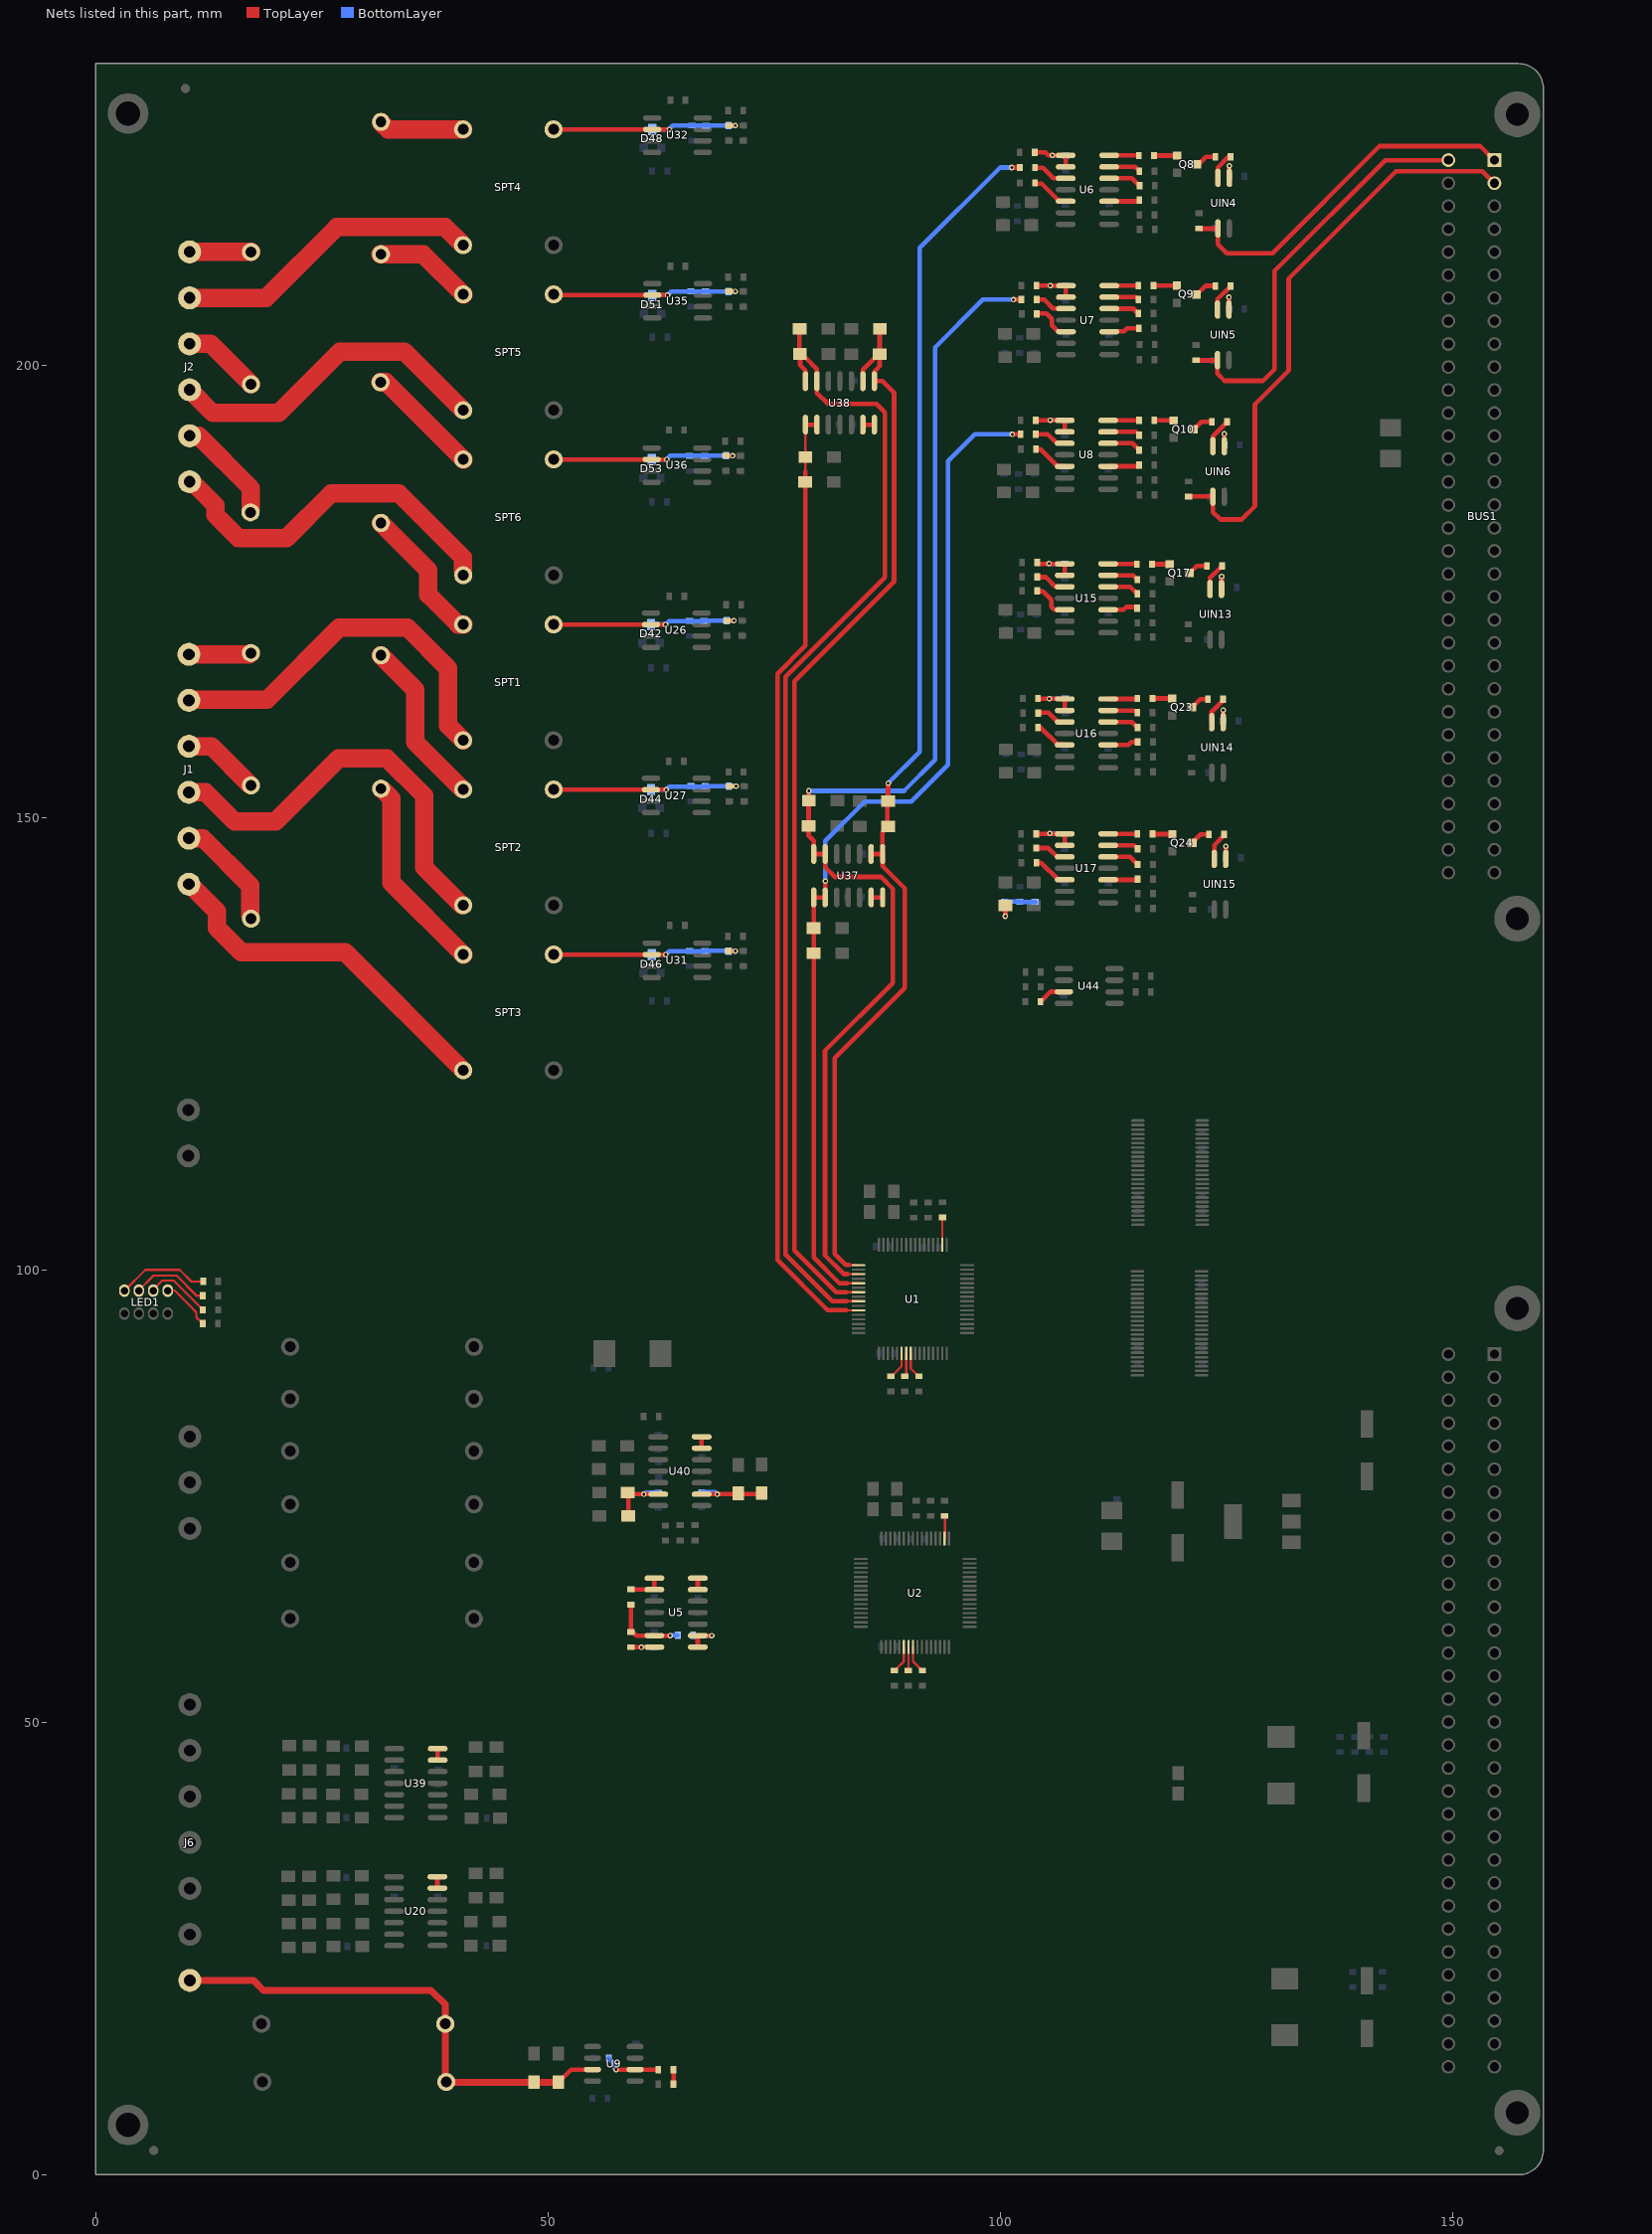
[diagram p0: the nets of this part, all layers, seen from the top]
# Altium PCB MISC80584.PCBDoc (part 6 of 7)
Units mm, origin at the board's own origin, x right, y up, seen from the top; angles counter-clockwise.
Board outline 160.02 x 233.3 mm, 4 copper layers (TopLayer, GND, POWER, BottomLayer); 386 components, 266 nets, 1374 pads, 640 vias.

## Via types
v1: diameter 0.61, hole 0.305, TopLayer to BottomLayer, 342 vias
v2: diameter 0.762, hole 0.381, TopLayer to BottomLayer, 197 vias
v3: diameter 0.508, hole 0.254, TopLayer to BottomLayer, 101 vias

## Nets (pads, with @x,y where several pads share a name; then routed paths per layer and width w, separated by ;. In a path a pad name is that pad's centre, name@x,y a point inside that pad or via, vN(x,y) a via of type N, cw(c..) or ccw(c..) an arc to the next point about the centre after c; other vN are vias at no path point) (continued)
NetD91_A: D91.A R359.1 R366.2 R374.2 | length 6.2
  TopLayer w0.508: v1(100.559,139.116) D91.A@100.559,140.284
  BottomLayer w0.508: v1@100.559,139.167 100.559,140.64 R359.1@100.482,140.716 R374.2@102.159,140.716 102.184,140.716 102.235,140.665 R366.2@103.886,140.665
NetD94_A: D94.A D96.K R93.2 U40.6 | length 7.1
  TopLayer w0.508: D94.A@58.903,73.05 58.903,75.159 59.004,75.26 59.03,75.235 60.528,75.235 v1(60.604,75.235) U40.6@62.192,75.235
  BottomLayer w0.508: v1@60.63,75.235 60.808,75.413 R93.2@62.179,75.413
NetD95_A: D95.A D97.K R85.2 U40.9 | length 8.4
  TopLayer w0.508: U40.9@66.992,75.235 v1(68.707,75.235) ; v1@68.758,75.235 D97.K@73.635,75.235
  BottomLayer w0.508: R85.2@67.005,75.463 68.453,75.463 v1@68.707,75.209
NetLED1_1: LED1.1 R339.1 | length 10.1
  TopLayer w0.254: LED1.1@3.175,97.739 3.226,97.739 5.512,100.025 9.296,100.025 10.592,98.73 R339.1@11.836,98.73
NetLED1_3: LED1.3 R342.1 | length 8.8
  TopLayer w0.254: LED1.3@4.674,97.663 6.401,99.39 8.966,99.39 11.201,97.155 R342.1@11.811,97.155
NetLED1_5: LED1.5 R340.1 | length 6.9
  TopLayer w0.254: LED1.5@6.477,97.942 7.379,98.844 8.623,98.844 R340.1@11.735,95.733
NetLED1_7: LED1.7 R341.1 | length 5.7
  TopLayer w0.254: LED1.7@7.975,97.739 8.738,97.739 10.389,96.088 11.138,95.339 11.138,94.78 11.76,94.158 R341.1@11.76,94.056
NetQ8_B: Q8.B R162.1 | length 2.4
  TopLayer w0.508: R162.1@117.145,223.164 Q8.B@119.558,223.164
NetQ8_C: Q8.C R491.2 | length 2.1
  TopLayer w0.508: Q8.C@121.996,222.301 122.733,223.037 R491.2@123.774,223.037
NetQ9_B: Q9.B R211.1 | length 2.5
  TopLayer w0.508: R211.1@116.992,208.788 Q9.B@119.507,208.788
NetQ9_C: Q9.C R492.2 | length 2.2
  TopLayer w0.508: Q9.C@121.92,208.001 122.682,208.763 R492.2@123.774,208.763
NetQ10_B: Q10.B R225.1 | length 1.9
  TopLayer w0.508: R225.1@117.018,193.904 Q10.B@118.923,193.904
NetQ10_C: Q10.C R493.2 | length 2.3
  TopLayer w0.508: Q10.C@121.437,192.938 122.225,193.726 R493.2@123.393,193.726
NetQ17_B: Q17.B R382.1 | length 1.8
  TopLayer w0.508: R382.1@116.764,178.003 Q17.B@118.542,178.003
NetQ17_C: Q17.C R510.2 | length 1.9
  TopLayer w0.508: Q17.C@121.133,177.241 121.717,177.825 R510.2@122.834,177.825
NetQ23_B: Q23.B R383.1 | length 2.1
  TopLayer w0.508: R383.1@116.865,163.144 116.891,163.17 Q23.B@118.999,163.17
NetQ23_C: Q23.C R511.2 | length 1.9
  TopLayer w0.508: Q23.C@121.387,162.382 122.098,163.093 R511.2@122.961,163.093
NetQ24_B: Q24.B R384.1 | length 2.1
  TopLayer w0.508: R384.1@116.967,148.184 Q24.B@119.024,148.184
NetQ24_C: Q24.C R512.2 | length 2.3
  TopLayer w0.508: Q24.C@121.183,147.218 122.123,148.158 123.012,148.158 R512.2@123.063,148.107
NetR10_1: R10.1 R12.1 R13.2 U5.6 | length 8
  TopLayer w0.508: R13.2@59.182,60.02 R10.1@59.182,62.916 ; R13.2@59.36,60.02 59.766,59.614 U5.6@61.76,59.614 v1(63.5,59.614)
  BottomLayer w0.508: v1(63.5,59.614) 63.525,59.639 R12.1@64.313,59.639
NetR10_2: R10.2 U5.1 U5.2 | length 3.7
  TopLayer w0.508: R10.2@59.233,64.694 U5.2@61.76,64.694 U5.1@61.76,65.824
NetR11_1: R11.1 R14.2 U9.6 | length 6.2
  TopLayer w0.508: v1(57.531,11.659) U9.6@59.627,11.659 R14.2@62.103,11.659
  BottomLayer w0.508: R11.1@56.693,12.929 57.379,12.243 57.379,11.811 v1(57.531,11.659)
NetR12_2: R12.2 U5.8 U5.9 | length 4.6
  TopLayer w0.508: U5.8@66.56,58.344 U5.9@66.56,59.448 ; U5.9@66.56,59.614 v1(68.097,59.614)
  BottomLayer w0.508: R12.2@66.167,59.614 66.192,59.588 68.123,59.588 v1(68.097,59.614)
NetR13_1: R13.1 R28.2 U5.7 | length 3.3
  TopLayer w0.508: R13.1@59.182,58.344 U5.7@61.036,58.344
  BottomLayer w0.508: v1(60.325,58.318) 60.35,58.344 R28.2@61.747,58.344
NetR33_1: R33.1 U1.34 | length 2.8
  TopLayer w0.254: U1.34@93.589,102.805 R33.1@93.589,105.603
NetR34_1: R34.1 U2.34 | length 2.5
  TopLayer w0.254: U2.34@93.843,70.344 93.891,70.392 93.891,72.763 R34.1@93.843,72.811
NetR37_1: R37.1 U6.3 | length 3.7
  TopLayer w0.508: R37.1@103.962,221.818 104.699,221.818 105.867,220.65 U6.3@107.226,220.65
NetR40_1: R40.1 U7.3 | length 3
  TopLayer w0.508: R40.1@104.013,207.239 104.851,207.239 105.816,206.273 U7.3@106.578,206.273
NetR48_1: R48.1 U8.3 | length 3.5
  TopLayer w0.508: R48.1@104.013,192.38 105.232,192.38 106.248,191.364 U8.3@107.125,191.364
NetR57_2: R57.2 R76.2 U6.1 U6.2 | length 6.1
  TopLayer w0.508: R57.2@103.861,223.52 104.978,223.52 105.308,223.19 v1(105.766,223.19) 105.791,223.19 107.087,223.19 107.226,223.05 U6.2@107.226,221.92
  BottomLayer w0.508: v1(105.766,223.19) R76.2@107.188,223.19
NetR58_2: R58.2 R86.2 U7.1 U7.2 | length 6.1
  TopLayer w0.508: R58.2@103.988,208.839 104.038,208.788 v1(105.512,208.788) U7.1@107.252,208.788 ; U7.1@107.239,208.737 107.252,208.725 U7.2@107.252,207.518
  BottomLayer w0.508: v1@105.613,208.788 R86.2@107.213,208.788
NetR59_2: R59.2 R87.2 U8.1 U8.2 | length 5.9
  TopLayer w0.508: R59.2@104.115,193.904 v1@105.512,193.904 ; v1(105.512,193.929) v1@105.512,193.904 ; U8.2@107.125,192.634 U8.1@107.125,193.814 ; U8.1@107.125,193.904 v1@105.512,193.904
  BottomLayer w0.508: v1@105.588,193.904 R87.2@107.112,193.904 R87.2@107.239,193.904
NetR145_1: R145.1 SPT1.0 | length 15.3
  TopLayer w2.032: R145.1@31.545,182.565 36.779,177.33 36.779,174.65 40.081,171.348 SPT1.0@40.665,171.348
NetR150_1: R150.1 U6.13 | length 3.5
  TopLayer w0.508: U6.13@112.026,221.92 114.884,221.92 R150.1@115.341,221.463
NetR151_1: R151.1 U7.13 | length 3.3
  TopLayer w0.508: U7.13@112.052,207.518 114.986,207.518 R151.1@115.214,207.289
NetR152_1: R152.1 U8.13 | length 3.6
  TopLayer w0.508: U8.13@111.925,192.634 115.011,192.634 R152.1@115.367,192.278
NetR155_1: R155.1 U6.12 | length 3.6
  TopLayer w0.508: U6.12@112.026,220.65 114.554,220.65 R155.1@115.316,219.888
NetR156_1: R156.1 U7.12 | length 3.3
  TopLayer w0.508: U7.12@112.052,206.248 114.706,206.248 R156.1@115.164,205.791
NetR157_1: R157.1 U8.12 | length 3.6
  TopLayer w0.508: U8.12@111.925,191.364 114.605,191.364 R157.1@115.24,190.729
NetR161_1: R161.1 SPT2.0 | length 18.2
  TopLayer w2.032: R161.1@31.545,167.934 35.331,164.147 35.331,158.344 SPT2.0@40.335,153.34
NetR162_2: R162.2 U6.14 | length 3.2
  TopLayer w0.508: U6.14@112.026,223.19 R162.2@115.24,223.19
NetR165_1: R165.1 SPT3.0 | length 21.8
  TopLayer w2.032: R165.1@31.775,153.035 32.69,152.121 32.69,142.823 SPT3.0@40.64,134.872
NetR168_1: R168.1 SPT4.0 | length 9.3
  TopLayer w2.032: R168.1@31.598,226.771 32.31,226.058 SPT4.0@40.615,226.058
NetR171_1: R171.1 SPT5.0 | length 11
  TopLayer w2.032: R171.1@31.496,212.268 36.193,212.268 SPT5.0@40.64,207.821
NetR174_1: R174.1 SPT6.0 | length 12.7
  TopLayer w2.032: R174.1@31.471,198.12 32.104,198.12 SPT6.0@40.64,189.584
NetR211_2: R211.2 U7.14 | length 3.1
  TopLayer w0.508: U7.14@112.052,208.788 R211.2@115.164,208.788
NetR224_1: R224.1 U44.3 | length 2.8
  TopLayer w0.508: R224.1@104.597,129.819 105.537,130.759 U44.3@107.036,130.759
NetR225_2: R225.2 U8.14 | length 3.3
  TopLayer w0.508: U8.14@111.925,193.904 R225.2@115.265,193.904
NetR349_1: R349.1 U15.3 | length 3.5
  TopLayer w0.508: R349.1@104.089,176.581 105.029,176.581 106.096,175.514 U15.3@107.125,175.514
NetR350_1: R350.1 U16.3 | length 3.1
  TopLayer w0.508: R350.1@104.496,161.595 105.334,161.595 106.35,160.579 U16.3@107.125,160.579
NetR351_1: R351.1 U17.3 | length 3.4
  TopLayer w0.508: R351.1@104.14,146.634 105.308,146.634 106.274,145.669 U17.3@107.125,145.669
NetR353_2: R353.2 R360.2 U15.1 U15.2 | length 5.9
  TopLayer w0.508: R353.2@104.038,178.054 v1@105.385,178.054 ; v1(105.385,178.079) v1@105.385,178.054 ; U15.2@107.125,176.784 U15.1@107.125,177.965 ; U15.1@107.125,178.054 v1@105.385,178.054
  BottomLayer w0.508: v1@105.512,178.054 R360.2@107.112,178.054
NetR354_2: R354.2 R361.2 U16.1 U16.2 | length 5.5
  TopLayer w0.508: R354.2@104.369,163.144 v1(105.41,163.144) 105.537,163.144 U16.1@106.731,163.144 ; U16.1@106.731,163.119 U16.1@107.125,163.119 U16.2@107.125,161.912
  BottomLayer w0.508: v1(105.41,163.144) R361.2@106.985,163.144
NetR355_2: R355.2 R362.2 U17.1 U17.2 | length 5.8
  TopLayer w0.508: R355.2@104.178,148.221 v1@105.486,148.221 ; v1(105.486,148.26) v1@105.486,148.221 ; U17.2@107.125,146.939 U17.1@107.125,148.209 107.125,148.221 v1@105.486,148.221
  BottomLayer w0.508: v1(105.486,148.26) R362.2@107.01,148.26
NetR375_1: R375.1 U15.13 | length 3.4
  TopLayer w0.508: U15.13@111.925,176.784 114.681,176.784 R375.1@115.113,176.352
NetR376_1: R376.1 U16.13 | length 3.2
  TopLayer w0.508: U16.13@111.925,161.849 114.757,161.849 R376.1@115.011,161.595
NetR377_1: R377.1 U17.13 | length 3.4
  TopLayer w0.508: U17.13@111.925,146.939 114.757,146.939 R377.1@115.138,146.558
NetR379_1: R379.1 U15.12 | length 3.5
  TopLayer w0.508: U15.12@111.925,175.514 114.351,175.514 R379.1@115.087,174.777
NetR380_1: R380.1 U16.12 | length 3.3
  TopLayer w0.508: U16.12@111.925,160.579 114.554,160.579 R380.1@115.062,160.071
NetR381_1: R381.1 U17.12 | length 3.6
  TopLayer w0.508: U17.12@111.925,145.669 114.325,145.669 R381.1@115.138,144.856
NetR382_2: R382.2 U15.14 | length 3
  TopLayer w0.508: U15.14@111.925,178.054 R382.2@114.91,178.054
NetR383_2: R383.2 U16.14 | length 3.2
  TopLayer w0.508: U16.14@111.925,163.119 115.087,163.119 R383.2@115.113,163.144
NetR384_2: R384.2 U17.14 | length 3.1
  TopLayer w0.508: U17.14@111.925,148.209 R384.2@115.037,148.209
NetR399_1: R399.1 U6.5 | length 4.1
  TopLayer w0.508: R399.1@103.911,220.04 104.572,220.04 106.502,218.11 U6.5@107.226,218.11
NetR400_1: R400.1 U7.5 | length 4.5
  TopLayer w0.508: R400.1@103.988,205.74 104.013,205.715 105.105,205.715 105.689,205.13 105.689,204.419 106.401,203.708 U7.5@107.252,203.708
NetR401_1: R401.1 U8.5 | length 3.8
  TopLayer w0.508: R401.1@104.089,190.729 104.445,190.729 106.324,188.849 U8.5@107.086,188.849 ; U8.5@107.086,188.824 U8.5@107.125,188.824
NetR423_1: R423.1 U15.5 | length 4.3
  TopLayer w0.508: R423.1@104.064,175.031 R423.1@104.191,175.031 ; R423.1@104.191,174.955 R423.1@104.216,174.955 ; R423.1@104.216,175.006 104.724,175.006 105.644,174.086 105.644,173.324 105.994,172.974 U15.5@107.125,172.974
NetR430_1: R430.1 U16.5 | length 3.7
  TopLayer w0.508: R430.1@104.292,159.995 104.394,159.995 105.435,158.953 105.461,158.953 106.35,158.064 U16.5@107.188,158.064
NetR431_1: R431.1 U17.5 | length 3.9
  TopLayer w0.508: R431.1@104.064,145.009 R431.1@104.089,145.009 ; R431.1@104.089,145.034 104.496,145.034 106.401,143.129 U17.5@107.125,143.129
NetR435_1: R435.1 U8.10 | length 3.3
  TopLayer w0.508: U8.10@111.925,188.824 R435.1@115.24,188.824
NetR437_1: R437.1 U6.10 | length 3.3
  TopLayer w0.508: U6.10@112.026,218.11 R437.1@115.316,218.11
NetR438_1: R438.1 U7.10 | length 3.4
  TopLayer w0.508: U7.10@112.052,203.708 112.077,203.733 113.665,203.733 113.995,204.064 R438.1@115.291,204.064
NetR444_1: R444.1 U15.10 | length 3.3
  TopLayer w0.508: U15.10@111.925,172.974 113.64,172.974 113.944,173.279 R444.1@115.113,173.279
NetR445_1: R445.1 U16.10 | length 3.4
  TopLayer w0.508: U16.10@111.925,158.039 114.148,158.039 114.478,158.369 R445.1@115.189,158.369
NetR446_1: R446.1 U17.10 | length 3.2
  TopLayer w0.508: U17.10@111.925,143.129 R446.1@115.087,143.129
NetR486_2: R486.2 UIN4.1 | length 2.5
  TopLayer w0.508: UIN4.1@125.324,220.701 v1(125.324,222.047)
  BottomLayer w0.508: R486.2@125.324,220.929 v1(125.324,222.047)
NetR487_2: R487.2 UIN5.1 | length 2.6
  TopLayer w0.508: UIN5.1@125.273,206.146 v1(125.273,207.518)
  BottomLayer w0.508: v1@125.273,207.467 125.273,206.248 R487.2@125.298,206.223
NetR488_2: R488.2 UIN6.1 | length 2.6
  TopLayer w0.508: UIN6.1@124.765,191.059 124.765,192.43 v1(124.765,192.405)
  BottomLayer w0.508: R488.2@124.739,191.313 124.765,191.338 124.765,192.43 v1(124.765,192.405)
NetR491_1: R491.1 UIN4.2 | length 3.1
  TopLayer w0.508: UIN4.2@124.054,220.701 124.054,221.844 125.273,223.063 R491.1@125.527,223.063
NetR492_1: R492.1 UIN5.2 | length 3
  TopLayer w0.508: UIN5.2@124.003,206.146 124.003,207.289 R492.1@125.349,208.636
NetR493_1: R493.1 UIN6.2 | length 3.4
  TopLayer w0.508: UIN6.2@123.495,191.059 123.495,192.13 125.09,193.726 R493.1@125.12,193.726
NetR503_2: R503.2 UIN13.1 | length 2.6
  TopLayer w0.508: UIN13.1@124.46,175.26 v1(124.46,176.657)
  BottomLayer w0.508: R503.2@124.46,175.463 v1(124.46,176.657)
NetR506_2: R506.2 UIN14.1 | length 2.6
  TopLayer w0.508: UIN14.1@124.638,160.553 v1(124.638,161.874)
  BottomLayer w0.508: v1(124.638,161.874) 124.638,160.68 R506.2@124.689,160.63
NetR507_2: R507.2 UIN15.1 | length 2.6
  TopLayer w0.508: UIN15.1@124.917,145.44 v1(124.917,146.837)
  BottomLayer w0.508: R507.2@124.917,145.618 v1(124.917,146.837)
NetR510_1: R510.1 UIN13.2 | length 2.8
  TopLayer w0.508: UIN13.2@123.19,175.26 123.19,176.505 R510.1@124.308,177.622
NetR511_1: R511.1 UIN14.2 | length 2.9
  TopLayer w0.508: UIN14.2@123.368,160.553 123.368,161.696 R511.1@124.638,162.966
NetR512_1: R512.1 UIN15.2 | length 2.9
  TopLayer w0.508: UIN15.2@123.647,145.44 123.647,146.964 R512.1@124.612,147.93
NetR605_1: R605.1 U1.8 | length 2.7
  TopLayer w0.254: U1.8@90.089,90.805 90.089,89.134 R605.1@90.805,88.417 ; R605.1@90.983,88.367 R605.1@90.983,88.417
NetR607_1: R607.1 U1.7 | length 2.5
  TopLayer w0.254: R607.1@89.56,88.341 89.589,88.369 U1.7@89.589,90.805
NetR608_1: R608.1 U1.6 | length 2.7
  TopLayer w0.254: R608.1@88.163,88.443 89.089,89.368 U1.6@89.089,90.805
NetR609_1: R609.1 U2.8 | length 2.9
  TopLayer w0.254: U2.8@90.343,58.344 90.343,56.774 R609.1@91.288,55.829
NetR611_1: R611.1 U2.7 | length 2.4
  TopLayer w0.254: R611.1@89.843,55.979 U2.7@89.843,58.344
NetR612_1: R612.1 U2.6 | length 2.8
  TopLayer w0.254: R612.1@88.443,55.88 89.343,56.78 U2.6@89.343,58.344
NetU5_13: U5.13 U5.14 | length 1.3
  TopLayer w0.508: U5.14@66.599,65.888 66.56,65.849 U5.13@66.56,64.694 U5.13@66.65,64.783
NetU20_13: U20.13 U20.14 | length 1.3
  TopLayer w0.508: U20.14@37.744,32.969 37.782,32.931 U20.13@37.782,31.699
NetU37_13: U37.13 U37.14 | length 1.3
  TopLayer w0.508: U37.13@85.725,141.186 86.931,141.186 U37.14@86.995,141.122
NetU38_13: U38.13 U38.14 | length 1.1
  TopLayer w0.508: U38.13@85.027,193.434 U38.14@86.081,193.434
NetU39_13: U39.13 U39.14 | length 1.2
  TopLayer w0.508: U39.14@37.77,47.041 37.808,47.003 U39.13@37.808,45.847
NetU40_13: U40.13 U40.14 | length 1
  TopLayer w0.508: U40.13@66.992,80.556 U40.14@66.992,81.585
U1+: J2.1 R168.2 | length 6.8
  TopLayer w2.032: J2.1@10.389,212.522 R168.2@17.196,212.522
U1-: J2.2 SPT4.1 | length 34
  TopLayer w2.032: J2.2@10.389,207.442 18.847,207.442 26.67,215.265 38.633,215.265 SPT4.1@40.437,213.462
U1I: D10.A D14.K U1.55 U38.1 U38.2 | length 120.1
  TopLayer w0.254: 82.956,97.555 U1.55@84.339,97.555
  TopLayer w0.508: 82.956,97.561 81.864,97.561 77.241,102.184 77.241,165.075 88.265,176.098 88.265,196.926 86.957,198.234 U38.1@86.081,198.234 86.081,199.314 86.665,199.898 D10.A@86.665,201.219 86.665,203.784 D14.K@86.792,203.911 ; U38.2@84.811,198.234 84.811,199.517 D10.A@86.081,200.787
U1IN: C104.2 D48.3 R118.2 R119.2 R120.2 SPT4.3 U32.2 | length 22.7
  TopLayer w0.508: SPT4.3@50.597,226.06 U32.2@61.519,226.06 v1(63.424,226.06) ; C104.2@69.977,226.492 v1(70.714,226.492)
  BottomLayer w0.508: D48.3@61.544,226.06 63.373,226.06 63.779,226.466 R119.2@67.488,226.466 69.825,226.466 R118.2@69.85,226.492 ; R118.2@70.053,226.492 v1(70.714,226.492)
U2+: J2.3 R171.2 | length 8.6
  TopLayer w2.032: J2.3@10.389,202.362 12.725,202.362 R171.2@17.145,197.942
U2-: J2.4 SPT5.1 | length 36.6
  TopLayer w2.032: J2.4@10.389,197.282 12.954,194.716 20.218,194.716 27,201.498 34.138,201.498 SPT5.1@40.462,195.174
U2I: D24.A D29.K U1.57 U38.6 U38.7 | length 126.4
  TopLayer w0.254: 83.033,96.555 U1.57@84.339,96.555
  TopLayer w0.508: D29.K@77.775,201.397 77.775,203.962 D24.A@77.826,204.013 ; D29.K@77.876,201.066 77.876,200 78.461,199.415 U38.7@78.461,198.234 ; D29.K@78.384,200.914 79.731,199.568 U38.6@79.731,198.234 79.731,196.952 80.975,195.707 86.309,195.707 87.224,194.793 87.224,176.53 76.251,165.557 76.251,101.752 81.432,96.571 83.033,96.571
U2IN: C142.2 D51.3 R110.2 R111.2 R113.2 SPT5.3 U35.2 | length 21.9
  TopLayer w0.508: SPT5.3@51.003,207.747 U35.2@61.544,207.747 v1(63.221,207.747) ; C142.2@70.053,208.153 v1(70.714,208.153)
  BottomLayer w0.508: D51.3@61.798,207.747 v1(63.221,207.747) 63.627,208.153 R111.2@65.786,208.153 67.285,208.153 R110.2@67.31,208.178 ; R110.2@67.412,208.153 R113.2@69.952,208.153 v1(70.714,208.153)
U3+: J2.5 R174.2 | length 11.6
  TopLayer w2.032: J2.5@10.389,192.202 11.379,192.202 17.17,186.411 R174.2@17.17,183.998
U3-: J2.6 SPT6.1 | length 39.9
  TopLayer w2.032: J2.6@10.389,187.122 10.643,187.122 13.233,184.531 13.233,183.464 15.799,180.899 21.107,180.899 26.06,185.852 33.503,185.852 40.589,178.765 SPT6.1@40.589,177.241
U3I: D25.A D30.K U1.59 U38.8 U38.9 | length 106.2
  TopLayer w0.254: 78.461,188.239 D25.A@78.461,189.865 78.461,193.32 U38.8@78.461,193.434 ; 82.956,95.555 U1.59@84.339,95.555
  TopLayer w0.508: 78.461,188.239 78.461,169.012 75.362,165.913 75.362,101.117 80.899,95.58 82.956,95.58 ; U38.8@78.461,193.32 78.575,193.434 U38.9@79.731,193.434
U3IN: C130.2 D53.3 R105.2 R106.2 R414.2 SPT6.3 U36.2 | length 21.4
  TopLayer w0.508: SPT6.3@51.308,189.586 U36.2@61.468,189.586 v1(63.119,189.586) ; C130.2@69.672,190.017 70.434,190.017 70.434,189.992 v1(70.409,189.992)
  BottomLayer w0.508: D53.3@61.697,189.586 v1(63.119,189.586) 63.525,189.992 R105.2@65.659,189.992 67.183,189.992 R106.2@67.208,190.017 ; R106.2@67.361,189.992 R414.2@69.698,189.992 ; R414.2@69.748,189.992 69.774,190.017 70.434,190.017 70.434,189.992 v1(70.409,189.992)
UA: D8.A D12.K R37.2 U1.49 U37.1 U37.2 | length 136.7
  TopLayer w0.254: 83.287,100.555 U1.49@84.339,100.555 ; U37.2@85.725,145.948 85.763,145.986 85.776,145.999 86.411,145.999
  TopLayer w0.508: 83.287,100.559 82.906,100.559 81.686,101.778 81.686,123.419 89.459,131.191 89.459,142.189 86.995,144.653 U37.1@86.995,145.986 85.763,145.986 U37.2@85.725,145.986 ; U37.1@86.97,145.999 86.97,148.387 87.503,148.92 87.503,151.765 D12.K@87.63,151.892 ; D12.K@87.605,152.197 v1(87.605,153.797) ; v1(101.27,221.844) R37.2@102.159,221.844
  BottomLayer w0.508: v1(87.605,153.797) 91.084,157.277 91.084,212.954 99.974,221.844 v1(101.27,221.844)
UA+: J1.1 R145.2 | length 6.8
  TopLayer w2.032: J1.1@10.312,168.046 16.993,168.046 R145.2@17.094,168.148
UA-: J1.2 SPT1.1 | length 42.3
  TopLayer w2.032: J1.2@10.414,163.017 18.948,163.017 26.924,170.993 34.468,170.993 38.964,166.497 38.964,160.198 SPT1.1@40.615,158.547
UAIN: C82.2 D42.3 R137.2 R138.2 R139.2 SPT1.3 U26.2 | length 22
  TopLayer w0.508: SPT1.3@50.902,171.348 U26.2@61.392,171.348 v1(62.992,171.348) ; C82.2@69.774,171.78 v1(70.561,171.78)
  BottomLayer w0.508: D42.3@61.62,171.374 62.967,171.374 v1(62.992,171.348) 63.373,171.729 67.107,171.729 R139.2@67.183,171.806 ; R139.2@67.259,171.755 69.723,171.755 R137.2@69.748,171.78 ; R137.2@69.723,171.831 69.774,171.78 v1(70.561,171.78)
UB: D11.A D15.K R40.2 U1.51 U37.6 U37.7 | length 139.2
  TopLayer w0.254: 83.109,99.555 U1.51@84.339,99.555
  TopLayer w0.508: D11.A@78.842,151.867 v1(78.842,152.959) ; D11.A@78.918,151.74 78.816,151.638 D15.K@78.816,149.098 78.816,148.006 79.375,147.447 U37.7@79.375,145.986 80.632,145.986 U37.6@80.645,145.999 ; U37.6@80.645,145.986 80.645,144.501 81.686,143.459 86.792,143.459 88.113,142.138 88.113,131.724 80.62,124.231 80.62,101.625 82.677,99.568 83.109,99.568 ; v1(101.448,207.239) R40.2@102.337,207.239
  BottomLayer w0.508: v1(78.842,152.959) 89.357,152.959 92.786,156.388 92.786,201.955 98.069,207.239 v1(101.448,207.239)
UB+: J1.3 R161.2 | length 8.4
  TopLayer w2.032: J1.3@10.312,157.886 12.802,157.886 R161.2@16.993,153.695
UB-: J1.4 SPT2.1 | length 45.7
  TopLayer w2.032: J1.4@10.312,152.806 12.141,152.806 15.367,149.581 19.888,149.581 26.873,156.566 32.182,156.566 36.297,152.451 36.297,144.526 SPT2.1@40.462,140.36
UBIN: C88.2 D44.3 R130.2 R131.2 R133.2 SPT2.3 U27.2 | length 22.5
  TopLayer w0.508: SPT2.3@50.673,153.086 U27.2@61.392,153.086 v1(63.068,153.086) ; C88.2@70.104,153.467 v1(70.79,153.467)
  BottomLayer w0.508: D44.3@61.493,153.086 v1(63.068,153.086) 63.424,153.441 R133.2@67.386,153.441 ; R133.2@67.386,153.492 69.901,153.492 R130.2@69.926,153.467 ; R130.2@70.002,153.467 v1(70.79,153.467)
UC: D9.A D13.K R48.2 U1.53 U37.8 U37.9 | length 112.6
  TopLayer w0.254: U37.8@79.324,141.046 U37.8@79.35,141.021 ; 83.083,98.555 U1.53@84.339,98.555
  TopLayer w0.508: U37.9@80.67,141.249 80.607,141.186 U37.8@79.375,141.186 D9.A@79.375,137.795 D13.K@79.375,135.026 79.375,101.397 82.22,98.552 83.083,98.552 ; U37.9@80.67,141.91 v1(80.67,142.977) ; v1(101.321,192.354) R48.2@102.235,192.354
  BottomLayer w0.508: v1(80.67,142.977) 80.67,147.447 85.014,151.79 90.17,151.79 94.209,155.829 94.209,189.382 97.18,192.354 v1(101.321,192.354)
UC+: J1.5 R165.2 | length 12.2
  TopLayer w2.032: J1.5@10.312,147.726 11.862,147.726 17.094,142.494 R165.2@17.094,139.243
UC-: J1.6 SPT3.1 | length 39.7
  TopLayer w2.032: J1.6@10.312,142.646 10.389,142.646 13.411,139.624 13.411,137.82 16.104,135.128 27.584,135.128 SPT3.1@40.513,122.199
UCIN: C96.2 D46.3 R124.2 R125.2 R126.2 SPT3.3 U31.2 | length 21.9
  TopLayer w0.508: SPT3.3@51.13,134.899 51.156,134.874 U31.2@61.468,134.874 v1(63.017,134.874) ; C96.2@70.053,135.255 v1(70.714,135.255) ; v1(70.714,135.255) 70.739,135.255 70.739,135.28 v1(70.714,135.255)
  BottomLayer w0.508: D46.3@61.646,134.849 61.671,134.874 v1(63.017,134.874) 63.398,135.255 R125.2@67.259,135.255 ; R125.2@67.335,135.28 70.739,135.28 70.739,135.255 v1(70.714,135.255)
UPR1: BUS1.A1 R591.2 UIN4.3 | length 40.2
  TopLayer w0.508: R591.2@122.174,215.087 124.003,215.087 124.054,215.138 UIN4.3@124.054,215.113 124.054,213.36 125.044,212.369 130.073,212.369 141.91,224.206 147.193,224.206 153.06,224.206 BUS1.A1@154.61,222.656
UPR2: BUS1.C1 R592.2 UIN5.3 | length 45.9
  TopLayer w0.508: R592.2@121.818,200.533 123.952,200.533 124.003,200.482 124.003,199.06 124.79,198.272 129.057,198.272 130.327,199.542 130.327,210.414 142.57,222.656 146.253,222.656 BUS1.C1@149.53,222.656
UPR3: BUS1.A2 R593.2 UIN6.3 | length 65
  TopLayer w0.508: R593.2@120.929,185.496 123.368,185.496 123.495,185.623 UIN6.3@123.495,185.471 123.495,183.769 124.308,182.956 126.695,182.956 128.143,184.404 128.143,195.682 131.877,199.415 131.877,209.575 143.739,221.437 151.536,221.437 153.289,221.437 BUS1.A2@154.61,220.116
V16: C9.2 R14.1 | length 1.4
  TopLayer w0.508: R14.1@63.881,11.659 63.881,10.312 C9.2@63.932,10.262
V16_IN: D1.K D2.A J6.7 R6.2 R7.2 U9.3 | length 53.3
  TopLayer w0.508: D1.K@51.41,10.516 52.553,11.659 U9.3@54.927,11.659
  TopLayer w0.762: J6.7@10.414,21.514 17.475,21.514 18.567,20.422 37.059,20.422 38.633,18.847 38.633,10.922 R7.2@38.506,10.795 ; R7.2@39.319,10.236 48.463,10.236 48.489,10.262 D1.K@51.156,10.262
pads on no net: BUS1.0 BUS2.0 BUS2.A9 BUS2.A10 BUS2.C9 BUS2.C10 U1.15 U2.15 U4.16 U4.17 U4.19 U4.20 U4.22 U4.23 U4.37 U4.38 U4.40 U9.1 U9.5 U9.8 U26.5 U27.5 U31.5 U32.5 U35.5 U36.5 U44.1 U44.5 U44.7 U44.8

## Polygon pours and split planes (outlines as drawn)
GND on TopLayer "Top Layer-No Net" (solid, remove dead copper): 141.605,194.412 141.605,192.278 141.783,192.1 141.961,191.922 142.672,191.922 144.704,191.922 144.958,192.176 145.11,192.329 145.11,193.243 145.11,195.301 145.694,195.885 146.253,196.444 149.784,196.444 155.702,196.444 155.931,196.672 156.108,196.85 156.108,197.155 156.108,215.392 155.727,215.773 155.651,215.849 154.94,215.849 146.329,215.849 143.129,212.649 141.605,211.125 141.605,194.437